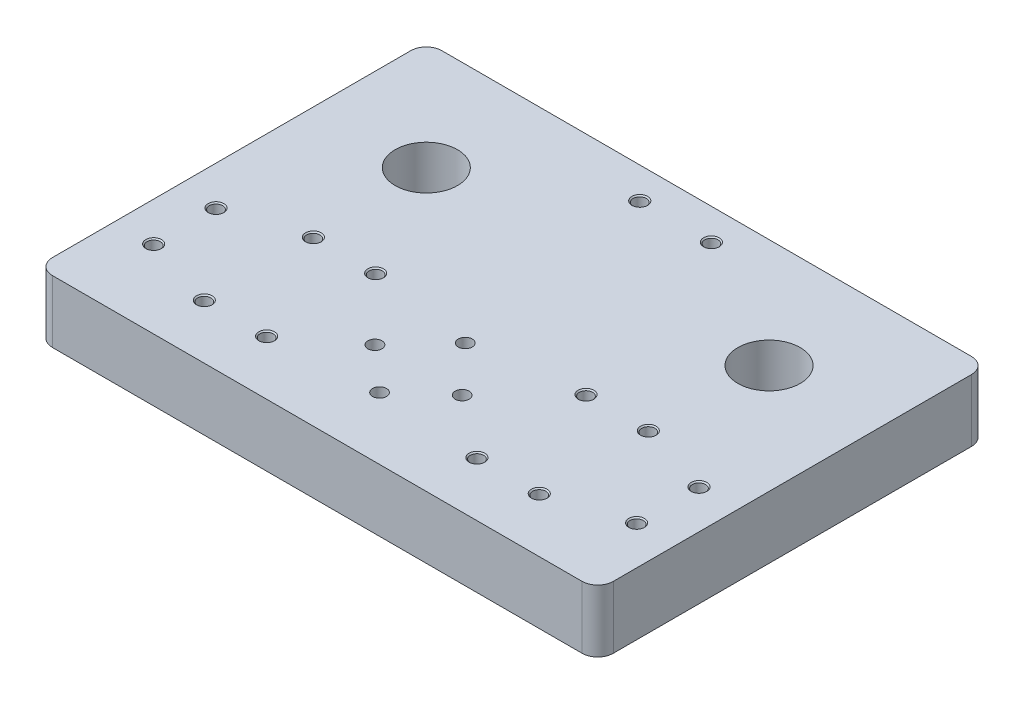
SolidWorks part; units mm, degrees
ref_plane "Front Plane" through (0, 0, 0) normal (0, 0, 1) x (1, 0, 0)
ref_plane "Top Plane" through (0, 0, 0) normal (0, 1, 0) x (1, 0, 0)
ref_plane "Right Plane" through (0, 0, 0) normal (1, 0, 0) x (0, 0, -1)
sketch "Sketch1" plane through (0, 0, 0) normal (0, 1, 0) x (1, 0, 0)
  line L0 (0, -1000) -> (0, 49000) construction
  line L1 (-170, -125) -> (170, -125)
  line L2 (-180, -115) -> (-180, 115)
  line L3 (-170, 125) -> (170, 125)
  line L4 (180, -115) -> (180, 115)
  line L5 (-180, -125) -> (180, 125) construction
  line L6 (-180, 125) -> (180, -125) construction
  arc A0 (-170, -125) -> (-180, -115) centre (-170, -115) cw
  arc A1 (170, -125) -> (180, -115) centre (170, -115) ccw
  arc A2 (170, 125) -> (180, 115) centre (170, 115) cw
  arc A3 (-180, 115) -> (-170, 125) centre (-170, 115) cw
  circle A4 centre (-110, 55) radius 20
  circle A5 centre (110, 55) radius 20
  circle A6 centre (0, -85) radius 4.5
  circle A7 centre (0, -30) radius 4.5
  circle A8 centre (28, -60) radius 4.5
  circle A9 centre (-28, -60) radius 4.5
  point P0 (0, 0)
  dimension "D3" = 10
  dimension "D4" = 40
  dimension "D5" = 40
  dimension "D6" = 70
  dimension "D7" = 70
  dimension "D8" = 110
  dimension "D9" = 110
  dimension "D10" = 9
  dimension "D11" = 9
  dimension "D12" = 40
  dimension "D13" = 95
  dimension "D14" = 9
  dimension "D15" = 9
  dimension "D16" = 65
  dimension "D17" = 65
  dimension "D18" = 28
  dimension "D19" = 28
  dimension "D1" = 360
  dimension "D2" = 250
extrude "Boss-Extrude1" add sketch "Sketch1" along normal blind 40
sketch "Sketch2" plane through (0, 0, 0) normal (0, -1, 0) x (1, 0, 0)
  circle A0 centre (0, 30) radius 7
  circle A1 centre (-28, 60) radius 7
  circle A2 centre (0, 85) radius 7
  circle A3 centre (28, 60) radius 7
  dimension "D1" = 14
  dimension "D2" = 14
  dimension "D3" = 14
  dimension "D4" = 14
extrude "Cut-Extrude1" cut sketch "Sketch2" against normal blind 9
hole_wizard "M10 Tapped Hole1" positions "Sketch3" profile "Sketch4" tap size "M10" standard "GB"
sketch "Sketch3" plane through (0, 40, 0) normal (0, 1, 0) x (1, 0, 0)
  line L0 (0, -1000) -> (0, 49000) construction
  line L1 (170, 125) -> (-170, 125) construction
  line L2 (-170, -125) -> (170, -125) construction
  point P0 (-23, 105)
  point P2 (-155, -35)
  point P4 (-155, -75)
  point P6 (-107.5, -20)
  point P8 (-67.5, -20)
  point P10 (-107.5, -90)
  point P12 (-67.5, -90)
  point P24 (155, -75)
  point P25 (155, -35)
  point P26 (67.5, -90)
  point P27 (107.5, -90)
  point P28 (67.5, -20)
  point P29 (107.5, -20)
  point P30 (23, 105)
  dimension "D1" = 23
  dimension "D2" = 20
  dimension "D3" = 105
  dimension "D4" = 105
  dimension "D5" = 90
  dimension "D6" = 50
  dimension "D7" = 35
  dimension "D8" = 35
  dimension "D9" = 67.5
  dimension "D10" = 67.5
  dimension "D11" = 107.5
  dimension "D12" = 107.5
  dimension "D13" = 155
  dimension "D14" = 155
sketch "Sketch4" plane through (-23, 40, -105) normal (1, 0, 0) x (0, 0, 1)
  line L0 (0, 0) -> (0, 30.0537)
  line L1 (0, 30.0537) -> (4.25, 27.5)
  line L2 (4.25, 27.5) -> (4.25, 0.775)
  line L3 (4.25, 0.775) -> (5.025, 0)
  line L5 (5.025, 0) -> (0, 0)
  line L6 (-4.25, 0.775) -> (-5.025, 0) construction
  line L10 (0, 30.0537) -> (-4.25, 27.5) construction
  line L11 (0, -6.35) -> (0, 107.95) construction
  dimension "螺纹孔钻头直径" = 8.5
  dimension "螺纹孔钻头深度" = 27.5
  dimension "近端锥形沉头孔直径" = 10.05
  dimension "近端锥形沉头孔角度" = 90
  dimension "导头角度" = 118
cosmetic thread "Hole Thread Line 1" parameters "D1"=20, "D2"=10
cosmetic thread "Hole Thread Line 2" parameters "D1"=20, "D2"=10
cosmetic thread "Hole Thread Line 3" parameters "D1"=20, "D2"=10
cosmetic thread "Hole Thread Line 4" parameters "D1"=20, "D2"=10
cosmetic thread "Hole Thread Line 5" parameters "D1"=20, "D2"=10
cosmetic thread "Hole Thread Line 6" parameters "D1"=20, "D2"=10
cosmetic thread "Hole Thread Line 7" parameters "D1"=20, "D2"=10
cosmetic thread "Hole Thread Line 8" parameters "D1"=20, "D2"=10
cosmetic thread "Hole Thread Line 9" parameters "D1"=20, "D2"=10
cosmetic thread "Hole Thread Line 10" parameters "D1"=20, "D2"=10
cosmetic thread "Hole Thread Line 11" parameters "D1"=20, "D2"=10
cosmetic thread "Hole Thread Line 12" parameters "D1"=20, "D2"=10
cosmetic thread "Hole Thread Line 13" parameters "D1"=20, "D2"=10
cosmetic thread "Hole Thread Line 14" parameters "D1"=20, "D2"=10
